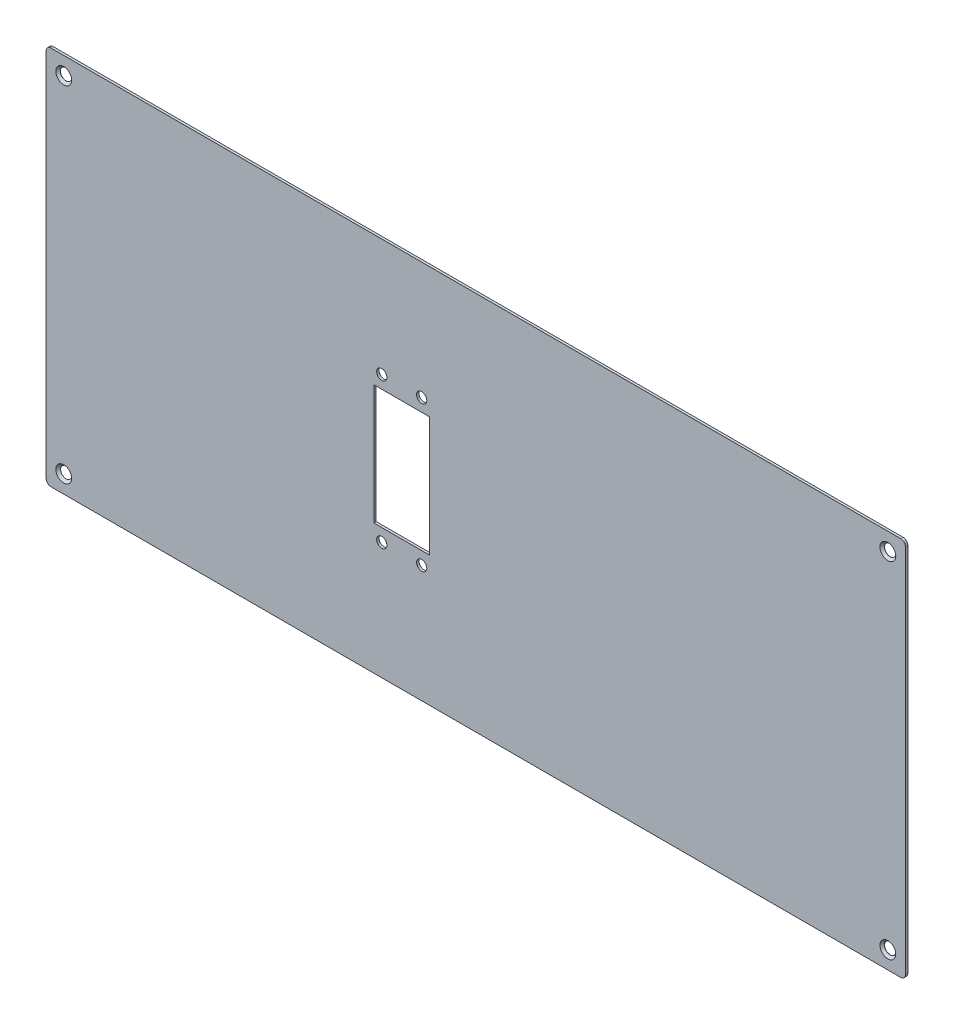
SolidWorks part; units mm, degrees
ref_plane "前视基准面" through (0, 0, 0) normal (0, 0, 1) x (1, 0, 0)
ref_plane "上视基准面" through (0, 0, 0) normal (0, 1, 0) x (1, 0, 0)
ref_plane "右视基准面" through (0, 0, 0) normal (1, 0, 0) x (0, 0, -1)
sketch "草图1" plane through (0, 0, 0) normal (0, 0, 1) x (1, 0, 0)
  line L0 (-232.6198, 20.5679) -> (305.5802, 20.5679)
  line L1 (305.5802, 20.5679) -> (305.5802, 258.5679)
  line L2 (305.5802, 258.5679) -> (-232.6198, 258.5679)
  line L3 (-232.6198, 258.5679) -> (-232.6198, 20.5679)
  dimension "D1" = 238
  dimension "D2" = 538.2
extrude "凸台-拉伸1" add sketch "草图1" against normal blind 1.5
hole_wizard "孔1" positions "草图3" profile "草图2" legacy
sketch "草图3" plane through (0, 0, 0) normal (0, 0, 1) x (1, 0, 0)
  line L0 (-232.6198, 20.5679) -> (305.5802, 20.5679) construction
  line L2 (-232.6198, 258.5679) -> (-232.6198, 20.5679) construction
  point P0 (-221.6198, 31.5679)
  dimension "D1" = 11
  dimension "D2" = 11
sketch "草图2" plane through (-221.6198, 31.5679, 0) normal (1, 0, 0) x (0, -1, 0)
  line L0 (0, 0) -> (0, 1.5)
  line L1 (0, 1.5) -> (3.45, 1.5)
  line L2 (3.45, 1.5) -> (4.95, 0)
  line L3 (4.95, 0) -> (0, 0)
  line L4 (0, 110) -> (0, -10) construction
  dimension "次要直径" = 6.9
  dimension "深度" = 1.5
  dimension "主要直径" = 9.9
hole_wizard "Ø7.1 (7.1) 直径孔1" positions "草图5" profile "草图4" hole size "Ø7.1" standard "ANSI Metric"
sketch "草图5" plane through (0, 0, 0) normal (0, 0, 1) x (1, 0, 0)
  line L0 (305.5802, 258.5679) -> (-232.6198, 258.5679) construction
  line L1 (305.5802, 20.5679) -> (305.5802, 258.5679) construction
  line L2 (-232.6198, 20.5679) -> (305.5802, 20.5679) construction
  line L3 (-232.6198, 258.5679) -> (-232.6198, 20.5679) construction
  point P0 (294.5802, 247.5679)
  point P1 (294.5802, 31.5679)
  point P2 (-221.6198, 247.5679)
  dimension "D1" = 11
  dimension "D2" = 11
  dimension "D3" = 11
  dimension "D4" = 11
  dimension "D5" = 11
  dimension "D6" = 11
sketch "草图4" plane through (294.5802, 247.5679, 0) normal (1, 0, 0) x (0, -1, 0)
  line L0 (0, 0) -> (0, 1.5)
  line L1 (0, 1.5) -> (3.55, 1.5)
  line L2 (3.55, 1.5) -> (3.55, 1.4)
  line L3 (3.55, 1.4) -> (4.95, 0)
  line L5 (4.95, 0) -> (0, 0)
  line L6 (-3.55, 1.4) -> (-4.95, 0) construction
  line L11 (0, -6.35) -> (0, 107.95) construction
  dimension "通孔孔直径" = 7.1
  dimension "通孔孔深度" = 1.5
  dimension "近端锥形沉头孔直径" = 9.9
  dimension "近端锥形沉头孔角度" = 90
fillet "圆角1" radius 3 4 edges at (305.5802, 20.5679, -0.75) (305.5802, 258.5679, -0.75) (-232.6198, 20.5679, -0.75) (-232.6198, 258.5679, -0.75)
sketch "草图6" plane through (0, 0, 0) normal (0, 0, 1) x (1, 0, 0)
  line L0 (305.5802, 23.5679) -> (305.5802, 255.5679) construction
  line L1 (7.5802, 102.0679) -> (-27.4198, 102.0679)
  line L2 (7.5802, 102.0679) -> (7.5802, 177.0679)
  line L3 (7.5802, 177.0679) -> (-27.4198, 177.0679)
  line L4 (-27.4198, 102.0679) -> (-27.4198, 177.0679)
  line L6 (-229.6198, 20.5679) -> (302.5802, 20.5679) construction
  dimension "D1" = 75
  dimension "D2" = 35
  dimension "D3" = 298
  dimension "D4" = 81.5
extrude "切除-拉伸1" cut sketch "草图6" against normal blind 1.5
sketch "草图7" plane through (0, 0, 0) normal (0, 0, 1) x (1, 0, 0)
  line L0 (-27.4198, 102.0679) -> (7.5802, 102.0679) construction
  line L1 (7.5802, 102.0679) -> (7.5802, 177.0679) construction
  circle A0 centre (2.5802, 94.0679) radius 3.2
  circle A1 centre (-22.4198, 94.0679) radius 3.2
  circle A2 centre (2.5802, 185.0679) radius 3.2
  circle A3 centre (-22.4198, 185.0679) radius 3.2
  dimension "D1" = 6.4
  dimension "D2" = 8
  dimension "D3" = 5
  dimension "D4" = 6.4
  dimension "D5" = 25
  dimension "D6" = 2
extrude "切除-拉伸2" cut sketch "草图7" against normal blind 1.5
